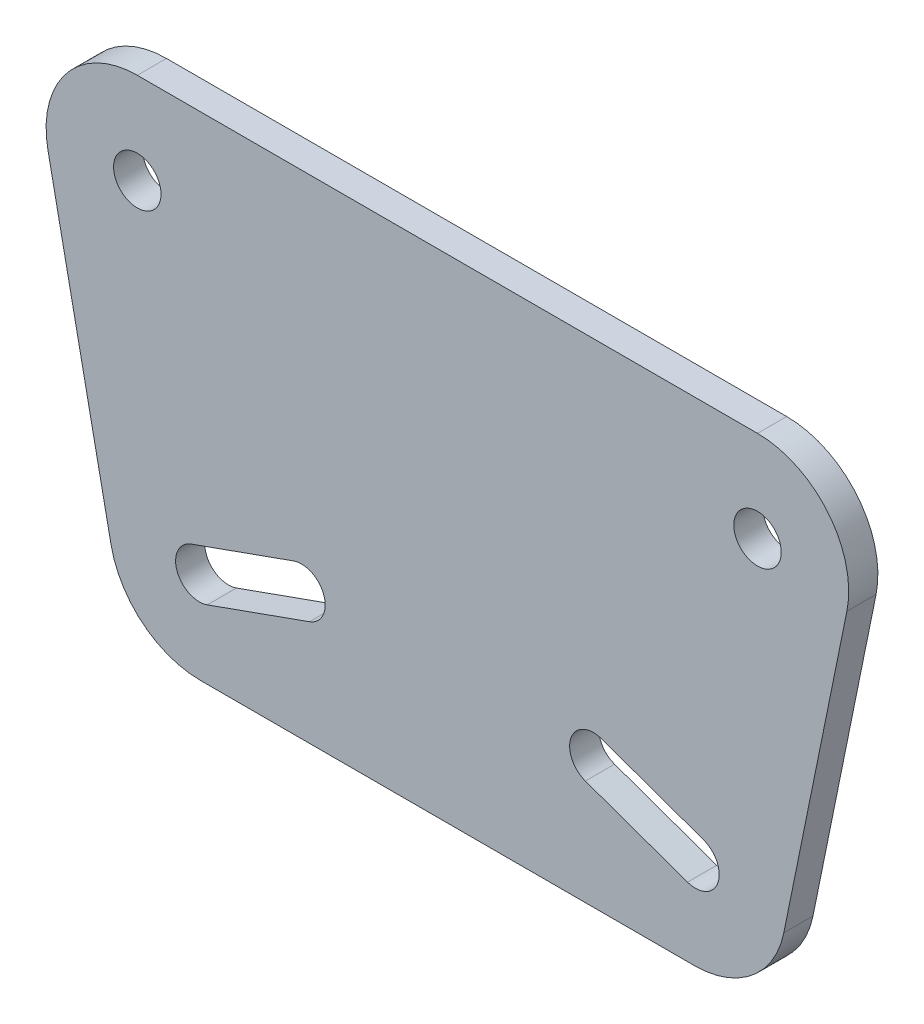
SolidWorks part; units mm, degrees
material "1023 Carbon steel plate (SS)"
ref_plane "Front Plane" through (0, 0, 0) normal (0, 0, 1) x (1, 0, 0)
ref_plane "Top Plane" through (0, 0, 0) normal (0, 1, 0) x (1, 0, 0)
ref_plane "Right Plane" through (0, 0, 0) normal (1, 0, 0) x (0, 0, -1)
sketch "Sketch1" plane through (0, 0, 0) normal (0, 0, 1) x (1, 0, 0)
  line L0 (0, 0) -> (170, 0)
  line L5 (-24.4981, -29.9842) -> (-7.2047, -114.9842)
  line L6 (194.4981, -29.9842) -> (177.2047, -114.9842)
  line L7 (17.2934, -135) -> (152.7066, -135)
  line L8 (-25, -25) -> (-25, -132.8689) construction
  line L9 (195, -25) -> (195, -145.0395) construction
  line L10 (17, -110) -> (45, -100) construction
  line L11 (14.8138, -103.8787) -> (42.8138, -93.8787)
  line L12 (19.1862, -116.1213) -> (47.1862, -106.1213)
  line L13 (85, 0) -> (85, -47.462) construction
  line L14 (125, -100) -> (153, -110) construction
  line L15 (127.1862, -93.8787) -> (155.1862, -103.8787)
  line L16 (122.8138, -106.1213) -> (150.8138, -116.1213)
  arc A0 (170, 0) -> (194.4981, -29.9842) centre (170, -25) cw
  arc A1 (0, 0) -> (-24.4981, -29.9842) centre (0, -25) ccw
  arc A2 (-7.2047, -114.9842) -> (17.2934, -135) centre (17.2934, -110) ccw
  arc A3 (177.2047, -114.9842) -> (152.7066, -135) centre (152.7066, -110) cw
  circle A4 centre (0, -25) radius 6.5
  arc A6 (14.8138, -103.8787) -> (19.1862, -116.1213) centre (17, -110) ccw
  arc A7 (47.1862, -106.1213) -> (42.8138, -93.8787) centre (45, -100) ccw
  circle A8 centre (170, -25) radius 6.5
  arc A9 (127.1862, -93.8787) -> (122.8138, -106.1213) centre (125, -100) ccw
  arc A10 (150.8138, -116.1213) -> (155.1862, -103.8787) centre (153, -110) ccw
  point P23 (31, -105)
  point P30 (139, -105)
  dimension "D3" = 25
  dimension "D1" = 25
  dimension "D2" = 25
  dimension "D4" = 25
  dimension "D7" = 13
  dimension "D11" = 6.5
  dimension "D16" = 13
  dimension "D17" = 6.5
  dimension "D5" = 135
  dimension "D6" = 220
  dimension "D8" = 28
  dimension "D9" = 45
  dimension "D10" = 40
  dimension "D12" = 10
  dimension "D13" = 75
  dimension "D14" = 100
  dimension "D15" = 23
  dimension "D18" = 10
  dimension "D19" = 28
  dimension "D20" = 40
  dimension "D21" = 45
extrude "Boss-Extrude1" add sketch "Sketch1" along normal blind 8 contours A4 | L16 A10 L15 A9 | L12 A7 L11 A6 | L7 A3 L6 A0 L0 A1 L5 A2 | A8
